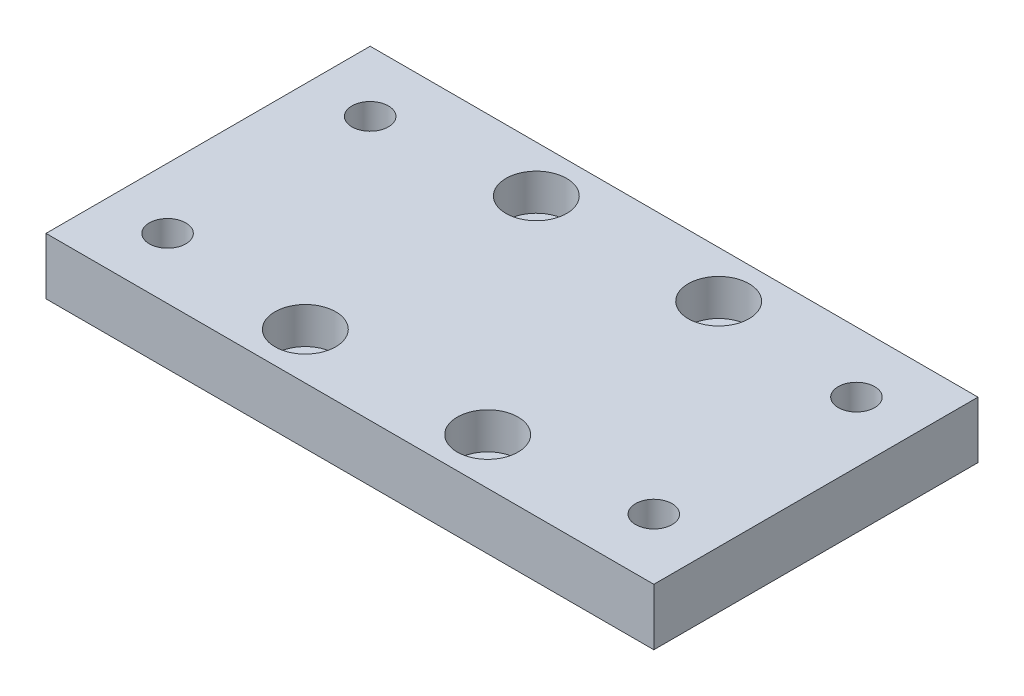
from build123d import *

# Parameters (mm, degrees)
SKETCH1_W                                         = 150
SKETCH1_H                                         = 80
BOSS_EXTRUDE1_DEPTH                               = 14
HOLE_SIZE_BY_SOCKET_HEAD_CAP_SCREW_TY_D           = 9
HOLE_SIZE_BY_SOCKET_HEAD_CAP_SCREW_TY_CBORE_D     = 15
HOLE_SIZE_BY_SOCKET_HEAD_CAP_SCREW_TY_CBORE_DEPTH = 9
F_9_0_9_DIAMETER_HOLE1_D                          = 9


with BuildPart() as part:
    # Sketch1 → Boss-Extrude1 (new body)
    with BuildSketch(Plane(origin=(0, 0, 0), x_dir=(1, 0, 0), z_dir=(0, 1, 0))):
        with Locations((75, 40)):
            Rectangle(SKETCH1_W, SKETCH1_H)
    extrude(amount=BOSS_EXTRUDE1_DEPTH)

    # Hole size (% by) socket head cap screw type1 (through all)
    with Locations(Plane(origin=(0, 14, 0), x_dir=(-1, 0, 0), z_dir=(0, 1, 0))):
        with Locations((-52.5, -68.5), (-52.5, -11.5), (-97.5, -11.5), (-97.5, -68.5)):
            CounterBoreHole(HOLE_SIZE_BY_SOCKET_HEAD_CAP_SCREW_TY_D / 2, HOLE_SIZE_BY_SOCKET_HEAD_CAP_SCREW_TY_CBORE_D / 2, HOLE_SIZE_BY_SOCKET_HEAD_CAP_SCREW_TY_CBORE_DEPTH)

    # Ø9.0 (9) Diameter Hole1 (through all)
    with Locations(Plane(origin=(0, 14, 0), x_dir=(-1, 0, 0), z_dir=(0, 1, 0))):
        with Locations((-15, -65), (-15, -15), (-135, -15), (-135, -65)):
            Hole(F_9_0_9_DIAMETER_HOLE1_D / 2)


solid = part.part
